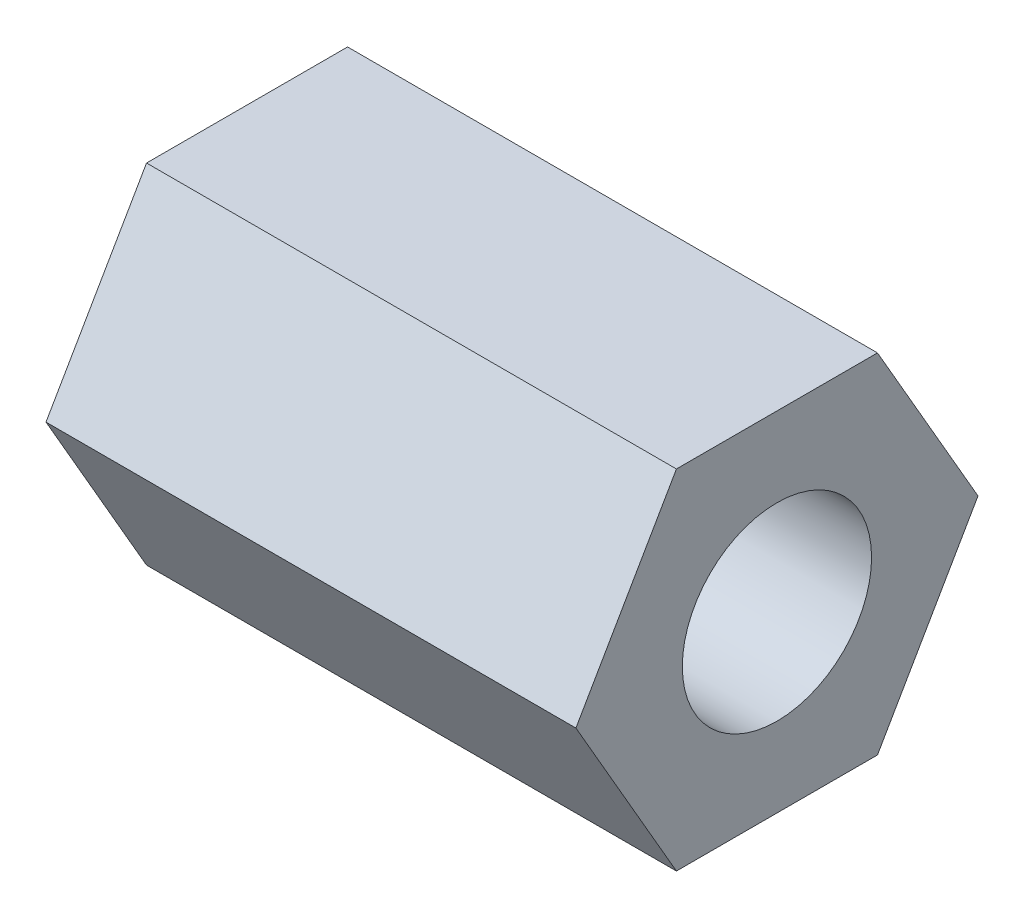
from build123d import *

# Parameters (mm, degrees)
EXTRUDE_1_DEPTH    = 7
HOLE_WIZARD_M3_1_D = 2.5


with BuildPart() as part:
    # 草图1 → 凸台-拉伸1 (new body)
    with BuildSketch(Plane(origin=(0, 0, 0), x_dir=(0, 0, -1), z_dir=(1, 0, 0))):
        Polygon((2.655811238, 0), (1.327905619, 2.3), (-1.327905619, 2.3), (-2.655811238, 0), (-1.327905619, -2.3), (1.327905619, -2.3), align=None)
    extrude(amount=EXTRUDE_1_DEPTH)

    # M3 螺纹孔1 (through all)
    with Locations(Plane(origin=(7, 0, 0), x_dir=(0, 0, -1), z_dir=(1, 0, 0))):
        with Locations((0, 0)):
            Hole(HOLE_WIZARD_M3_1_D / 2)


solid = part.part
